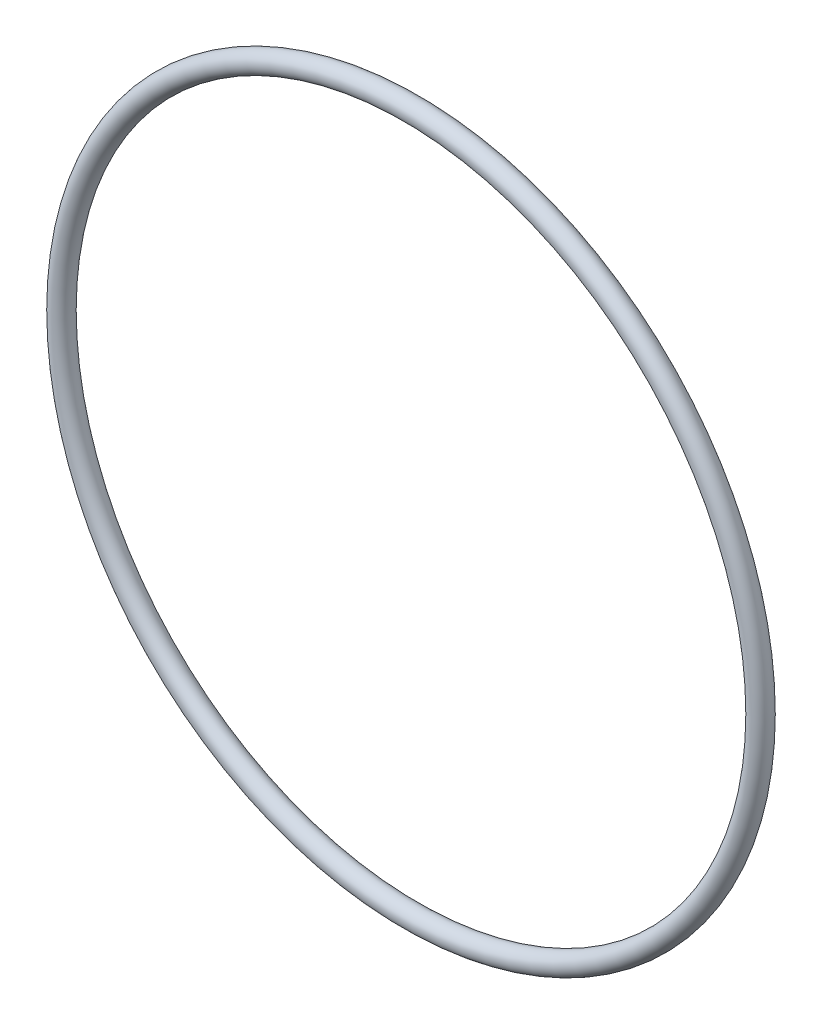
from build123d import *

# Parameters (mm, degrees)
SKETCH1_R = 1


with BuildPart() as part:
    # Sketch1 → Revolve1 (revolve)
    with BuildSketch(Plane(origin=(0, 0, 0), x_dir=(1, 0, 0), z_dir=(0, 1, 0))):
        with Locations((-33.5, 0)):
            Circle(SKETCH1_R)
    revolve(axis=Axis((0, 0, 0), (0, 0, 1)))


solid = part.part
